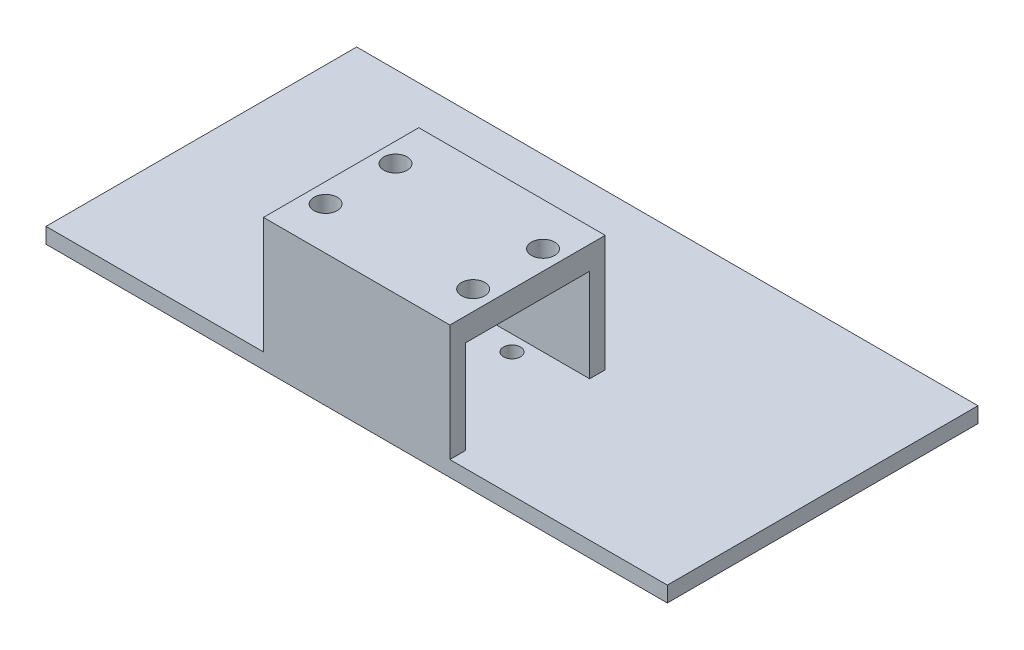
SolidWorks part; units mm, degrees
ref_plane "Front Plane" through (0, 0, 0) normal (0, 0, 1) x (1, 0, 0)
ref_plane "Top Plane" through (0, 0, 0) normal (0, 1, 0) x (1, 0, 0)
ref_plane "Right Plane" through (0, 0, 0) normal (1, 0, 0) x (0, 0, -1)
sketch "Sketch1" plane through (0, 0, 0) normal (0, 1, 0) x (1, 0, 0)
  line L1 (-40, -10) -> (40, -10)
  line L2 (-40, -10) -> (-40, 10)
  line L3 (-40, 10) -> (40, 10)
  line L4 (40, -10) -> (40, 10)
  line L5 (-40, -10) -> (40, 10) construction
  line L6 (-40, 10) -> (40, -10) construction
  circle A0 centre (-4, 6) radius 1.1
  circle A1 centre (4, 6) radius 1.1
  circle A2 centre (-4, -6) radius 1.1
  circle A3 centre (4, -6) radius 1.1
  point P0 (0, 0)
  dimension "D1" = 2.2
  dimension "D2" = 2.2
  dimension "D3" = 2.2
  dimension "D4" = 2.2
  dimension "D6" = 8
  dimension "D7" = 6
  dimension "D9" = 12
  dimension "D10" = 12
  dimension "D12" = 8
  dimension "D13" = 4
  dimension "D5" = 4
  dimension "D8" = 6
  dimension "D11" = 20
  dimension "D14" = 80
extrude "Boss-Extrude1" add sketch "Sketch1" along normal blind 2
sketch "Sketch3" plane through (0, 0, 0) normal (1, 0, 0) x (0, 0, -1)
  line L1 (-10, 2) -> (-8, 2)
  line L2 (-10, 2) -> (-10, 13.7829)
  line L4 (-8, 2) -> (-8, 14)
  line L5 (10, 2) -> (8, 2)
  line L6 (10, 2) -> (10, 13.7829)
  line L8 (8, 2) -> (8, 14)
  line L9 (-8, 14) -> (8, 14)
  line L10 (-10, 13.7829) -> (-10, 17)
  line L11 (-10, 17) -> (10, 17)
  line L12 (10, 13.7829) -> (10, 17)
  dimension "D1" = 12
  dimension "D2" = 3
  dimension "D3" = 2
  dimension "D4" = 2
extrude "Boss-Extrude3" add sketch "Sketch3" against normal mid plane 24
sketch "Sketch4" plane through (0, 17, 0) normal (0, 1, 0) x (1, 0, 0)
  circle A0 centre (9.5, -4.5) radius 1.5
  circle A1 centre (-9.5, -4.5) radius 1.5
  circle A2 centre (-9.5, 4.5) radius 1.5
  circle A3 centre (9.5, 4.5) radius 1.5
  dimension "D1" = 3
  dimension "D2" = 3
  dimension "D3" = 3
  dimension "D4" = 3
  dimension "D7" = 9
  dimension "D5" = 9
  dimension "D6" = 4.5
  dimension "D8" = 4.5
  dimension "D9" = 19
  dimension "D10" = 19
  dimension "D11" = 9.5
  dimension "D12" = 9.5
extrude "Cut-Extrude1" cut sketch "Sketch4" against normal blind 5
sketch "Sketch5" plane through (0, 0, -10) normal (0, 0, 1) x (1, 0, 0)
  line L0 (-40, 2) -> (-40, 0) construction
  line L1 (40, 0) -> (-40, 0)
  line L2 (40, 0) -> (40, 2)
  line L3 (40, 2) -> (-40, 2)
  line L4 (-40, 0) -> (-40, 2)
  dimension "D1" = 2
extrude "Boss-Extrude4" add sketch "Sketch5" against normal blind 20
